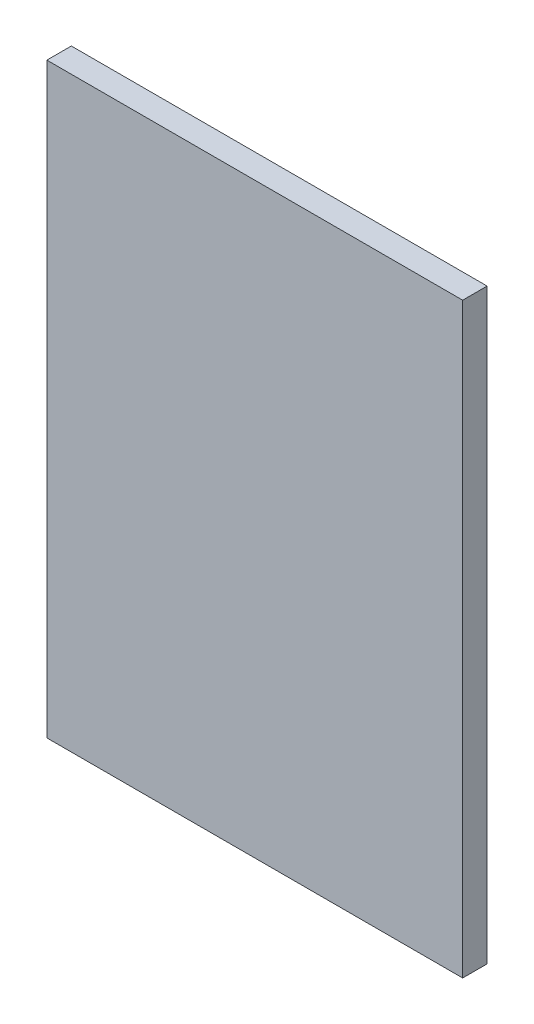
SolidWorks part; units mm, degrees
material "1023 碳钢板 (SS)"
ref_plane "前视基准面" through (0, 0, 0) normal (0, 0, 1) x (1, 0, 0)
ref_plane "上视基准面" through (0, 0, 0) normal (0, 1, 0) x (1, 0, 0)
ref_plane "右视基准面" through (0, 0, 0) normal (1, 0, 0) x (0, 0, -1)
sketch "草图1" plane through (0, 0, 0) normal (0, 0, 1) x (1, 0, 0)
  line L1 (85, 120) -> (-85, 120)
  line L2 (85, 120) -> (85, -120)
  line L3 (85, -120) -> (-85, -120)
  line L4 (-85, 120) -> (-85, -120)
  line L5 (85, 120) -> (-85, -120) construction
  line L6 (85, -120) -> (-85, 120) construction
  point P0 (0, 0)
  dimension "D1" = 170
  dimension "D2" = 240
extrude "凸台-拉伸1" add sketch "草图1" along normal blind 10
